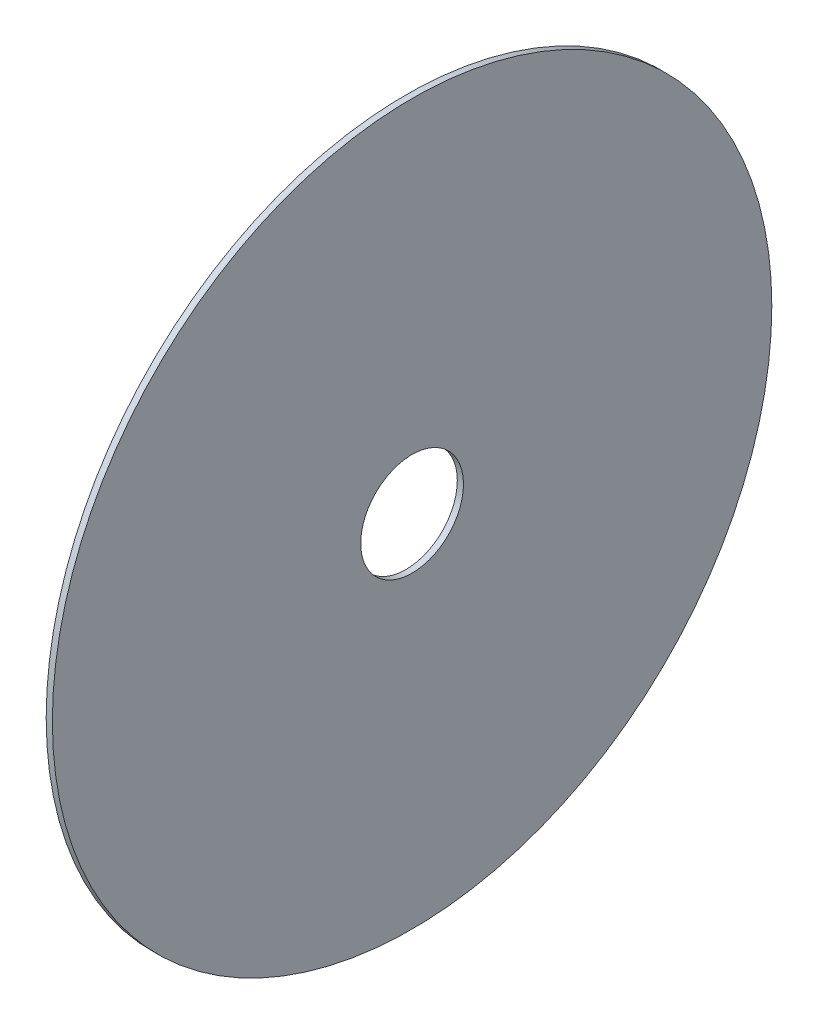
from build123d import *
from OCP.BRepFilletAPI import BRepFilletAPI_MakeChamfer

# Parameters (mm, degrees)
BOSS_EXTRUDE1_DEPTH = 4
CUT_EXTRUDE1_START  = -0.7
CUT_EXTRUDE1_DEPTH  = 0.7
CUT_EXTRUDE2_DEPTH  = 0.3
BOSS_EXTRUDE2_START = 0.3
BOSS_EXTRUDE2_DEPTH = 0.3
SKETCH5_W           = 3
SKETCH5_H           = 25
CHAMFER1_SIZE       = 1.130008551
CHAMFER1_SIZE2      = 0.565471506
SKETCH6_OUTSIDE_W   = 515.14
SKETCH6_OUTSIDE_H   = 515.14
SKETCH6_OUTSIDE_R   = 175
CUT_EXTRUDE3_DEPTH  = 10


with BuildPart() as part:
    # Sketch1 → Boss-Extrude1 (new body)
    with BuildSketch(Plane(origin=(-2, 0, 0), x_dir=(0, -1, 0), z_dir=(-1, 0, 0))):
        with BuildLine():
            Line((8.128598306, -199.834746453), (3.648717236, -192.075364828))
            ThreePointArc((3.648717236, -192.075364828), (3.941166203, -190.756212784), (5.280787083, -190.932577218))
            Line((5.280787083, -190.932577218), (12.558103906, -199.605345687))
            ThreePointArc((12.558103906, -199.605345687), (41.461654936, -195.655133258), (69.483089108, -187.54226278))
            Line((69.483089108, -187.54226278), (62.824688236, -181.547011706))
            ThreePointArc((62.824688236, -181.547011706), (62.695183332, -180.202051857), (64.023738106, -179.955818784))
            Line((64.023738106, -179.955818784), (73.624910537, -185.955297179))
            ThreePointArc((73.624910537, -185.955297179), (99.893138317, -173.266733442), (124.03609103, -156.891835741))
            Line((124.03609103, -156.891835741), (115.850941026, -153.247572166))
            ThreePointArc((115.850941026, -153.247572166), (115.312159093, -152.008458554), (116.499599564, -151.363730982))
            Line((116.499599564, -151.363730982), (127.48479795, -154.102648556))
            ThreePointArc((127.48479795, -154.102648556), (148.546385322, -133.917778536), (166.447576152, -110.883742691))
            Line((166.447576152, -110.883742691), (157.536896527, -109.947192524))
            ThreePointArc((157.536896527, -109.947192524), (156.641577295, -108.935218222), (157.571668516, -107.955106578))
            Line((157.571668516, -107.955106578), (168.8655851, -107.165358997))
            ThreePointArc((168.8655851, -107.165358997), (182.658877149, -81.460018407), (192.566012812, -54.021576334))
            Line((192.566012812, -54.021576334), (183.802042972, -55.88441563))
            ThreePointArc((183.802042972, -55.88441563), (182.637826525, -55.198639734), (183.219524688, -53.979084175))
            Line((183.219524688, -53.979084175), (193.716632226, -49.737977434))
            ThreePointArc((193.716632226, -49.737977434), (198.891445421, -21.028384111), (199.834746452, 8.128598305))
            Line((199.834746452, 8.128598305), (192.075364827, 3.648717235))
            ThreePointArc((192.075364827, 3.648717235), (190.756212783, 3.941166202), (190.932577217, 5.280787082))
            Line((190.932577217, 5.280787082), (199.605345686, 12.558103905))
            ThreePointArc((199.605345686, 12.558103905), (195.655133257, 41.461654935), (187.542262779, 69.483089106))
            Line((187.542262779, 69.483089106), (181.547011705, 62.824688235))
            ThreePointArc((181.547011705, 62.824688235), (180.202051856, 62.695183331), (179.955818783, 64.023738105))
            Line((179.955818783, 64.023738105), (185.955297178, 73.624910536))
            ThreePointArc((185.955297178, 73.624910536), (173.266733441, 99.893138316), (156.89183574, 124.036091029))
            Line((156.89183574, 124.036091029), (153.247572165, 115.850941024))
            ThreePointArc((153.247572165, 115.850941024), (152.008458553, 115.312159092), (151.363730981, 116.499599563))
            Line((151.363730981, 116.499599563), (154.102648555, 127.484797949))
            ThreePointArc((154.102648555, 127.484797949), (133.917778535, 148.546385321), (110.88374269, 166.447576151))
            Line((110.88374269, 166.447576151), (109.947192523, 157.536896526))
            ThreePointArc((109.947192523, 157.536896526), (108.935218221, 156.641577294), (107.955106577, 157.571668515))
            Line((107.955106577, 157.571668515), (107.165358996, 168.865585099))
            ThreePointArc((107.165358996, 168.865585099), (81.460018406, 182.658877148), (54.021576333, 192.566012811))
            Line((54.021576333, 192.566012811), (55.884415629, 183.802042971))
            ThreePointArc((55.884415629, 183.802042971), (55.198639733, 182.637826524), (53.979084174, 183.219524687))
            Line((53.979084174, 183.219524687), (49.737977433, 193.716632225))
            ThreePointArc((49.737977433, 193.716632225), (21.02838411, 198.89144542), (-8.128598306, 199.834746451))
            Line((-8.128598306, 199.834746451), (-3.648717236, 192.075364826))
            ThreePointArc((-3.648717236, 192.075364826), (-3.941166203, 190.756212782), (-5.280787083, 190.932577216))
            Line((-5.280787083, 190.932577216), (-12.558103906, 199.605345685))
            ThreePointArc((-12.558103906, 199.605345685), (-41.461654936, 195.655133256), (-69.483089107, 187.542262777))
            Line((-69.483089107, 187.542262777), (-62.824688236, 181.547011704))
            ThreePointArc((-62.824688236, 181.547011704), (-62.695183332, 180.202051855), (-64.023738106, 179.955818782))
            Line((-64.023738106, 179.955818782), (-73.624910537, 185.955297177))
            ThreePointArc((-73.624910537, 185.955297177), (-99.893138317, 173.26673344), (-124.03609103, 156.891835739))
            Line((-124.03609103, 156.891835739), (-115.850941025, 153.247572164))
            ThreePointArc((-115.850941025, 153.247572164), (-115.312159093, 152.008458552), (-116.499599564, 151.36373098))
            Line((-116.499599564, 151.36373098), (-127.48479795, 154.102648554))
            ThreePointArc((-127.48479795, 154.102648554), (-148.546385322, 133.917778533), (-166.447576152, 110.883742689))
            Line((-166.447576152, 110.883742689), (-157.536896527, 109.947192521))
            ThreePointArc((-157.536896527, 109.947192521), (-156.641577295, 108.93521822), (-157.571668516, 107.955106576))
            Line((-157.571668516, 107.955106576), (-168.8655851, 107.165358995))
            ThreePointArc((-168.8655851, 107.165358995), (-182.658877149, 81.460018404), (-192.566012812, 54.021576332))
            Line((-192.566012812, 54.021576332), (-183.802042972, 55.884415628))
            ThreePointArc((-183.802042972, 55.884415628), (-182.637826525, 55.198639732), (-183.219524688, 53.979084173))
            Line((-183.219524688, 53.979084173), (-193.716632226, 49.737977432))
            ThreePointArc((-193.716632226, 49.737977432), (-198.891445421, 21.028384109), (-199.834746452, -8.128598306))
            Line((-199.834746452, -8.128598306), (-192.075364827, -3.648717236))
            ThreePointArc((-192.075364827, -3.648717236), (-190.756212783, -3.941166203), (-190.932577217, -5.280787083))
            Line((-190.932577217, -5.280787083), (-199.605345686, -12.558103906))
            ThreePointArc((-199.605345686, -12.558103906), (-195.655133257, -41.461654937), (-187.542262778, -69.483089109))
            Line((-187.542262778, -69.483089109), (-181.547011705, -62.824688237))
            ThreePointArc((-181.547011705, -62.824688237), (-180.202051856, -62.695183333), (-179.955818783, -64.023738107))
            Line((-179.955818783, -64.023738107), (-185.955297178, -73.624910538))
            ThreePointArc((-185.955297178, -73.624910538), (-173.266733441, -99.893138318), (-156.89183574, -124.036091031))
            Line((-156.89183574, -124.036091031), (-153.247572165, -115.850941027))
            ThreePointArc((-153.247572165, -115.850941027), (-152.008458553, -115.312159094), (-151.363730981, -116.499599565))
            Line((-151.363730981, -116.499599565), (-154.102648555, -127.484797951))
            ThreePointArc((-154.102648555, -127.484797951), (-133.917778535, -148.546385324), (-110.88374269, -166.447576154))
            Line((-110.88374269, -166.447576154), (-109.947192522, -157.536896528))
            ThreePointArc((-109.947192522, -157.536896528), (-108.935218221, -156.641577296), (-107.955106577, -157.571668518))
            Line((-107.955106577, -157.571668518), (-107.165358996, -168.865585101))
            ThreePointArc((-107.165358996, -168.865585101), (-81.460018405, -182.65887715), (-54.021576333, -192.566012814))
            Line((-54.021576333, -192.566012814), (-55.884415629, -183.802042973))
            ThreePointArc((-55.884415629, -183.802042973), (-55.198639733, -182.637826526), (-53.979084174, -183.219524689))
            Line((-53.979084174, -183.219524689), (-49.737977433, -193.716632227))
            ThreePointArc((-49.737977433, -193.716632227), (-21.028384109, -198.891445422), (8.128598306, -199.834746453))
        make_face()
    extrude(amount=-BOSS_EXTRUDE1_DEPTH)

    # Sketch2 → Cut-Extrude1 (cut)
    with BuildSketch(Plane(origin=(2, 0, 0), x_dir=(0, 0, -1), z_dir=(1, 0, 0)).offset(CUT_EXTRUDE1_START)):
        with BuildLine():
            Line((181.547011705, -62.824688235), (181.845022607, -63.155662872))
            ThreePointArc((181.845022607, -63.155662872), (189.249413072, -35.226547542), (192.390100219, -6.503794095))
            Line((192.390100219, -6.503794095), (190.932577217, -5.280787082))
            ThreePointArc((190.932577217, -5.280787082), (190.756212783, -3.941166202), (192.075364827, -3.648717235))
            Line((192.075364827, -3.648717235), (192.461066825, -3.871402387))
            ThreePointArc((192.461066825, -3.871402387), (190.872489351, 24.978847229), (184.983641388, 53.266334763))
            Line((184.983641388, 53.266334763), (183.219524688, 53.979084175))
            ThreePointArc((183.219524688, 53.979084175), (182.637826525, 55.198639734), (183.802042972, 55.88441563))
            Line((183.802042972, 55.88441563), (184.237680867, 55.791817937))
            ThreePointArc((184.237680867, 55.791817937), (173.811636486, 82.739138395), (159.469694881, 107.822383645))
            Line((159.469694881, 107.822383645), (157.571668516, 107.955106578))
            ThreePointArc((157.571668516, 107.955106578), (156.641577295, 108.935218222), (157.536896527, 109.947192524))
            Line((157.536896527, 109.947192524), (157.979827047, 109.993746397))
            ThreePointArc((157.979827047, 109.993746397), (139.736889624, 132.400346217), (118.345743548, 151.824026374))
            Line((118.345743548, 151.824026374), (116.499599564, 151.363730982))
            ThreePointArc((116.499599564, 151.363730982), (115.312159093, 152.008458554), (115.850941025, 153.247572166))
            Line((115.850941025, 153.247572166), (116.257807045, 153.428720589))
            ThreePointArc((116.257807045, 153.428720589), (91.983722402, 169.101285665), (65.637286273, 180.964075582))
            Line((65.637286273, 180.964075582), (64.023738106, 179.955818784))
            ThreePointArc((64.023738106, 179.955818784), (62.695183332, 180.202051857), (62.824688236, 181.547011706))
            Line((62.824688236, 181.547011706), (63.155662873, 181.845022608))
            ThreePointArc((63.155662873, 181.845022608), (35.226547543, 189.249413073), (6.503794096, 192.39010022))
            Line((6.503794096, 192.39010022), (5.280787083, 190.932577218))
            ThreePointArc((5.280787083, 190.932577218), (3.941166203, 190.756212784), (3.648717236, 192.075364828))
            Line((3.648717236, 192.075364828), (3.871402389, 192.461066826))
            ThreePointArc((3.871402389, 192.461066826), (-24.978847228, 190.872489352), (-53.266334761, 184.983641389))
            Line((-53.266334761, 184.983641389), (-53.979084174, 183.219524689))
            ThreePointArc((-53.979084174, 183.219524689), (-55.198639733, 182.637826526), (-55.884415629, 183.802042973))
            Line((-55.884415629, 183.802042973), (-55.791817936, 184.237680869))
            ThreePointArc((-55.791817936, 184.237680869), (-82.739138394, 173.811636487), (-107.822383644, 159.469694882))
            Line((-107.822383644, 159.469694882), (-107.955106577, 157.571668518))
            ThreePointArc((-107.955106577, 157.571668518), (-108.935218221, 156.641577296), (-109.947192522, 157.536896528))
            Line((-109.947192522, 157.536896528), (-109.993746396, 157.979827048))
            ThreePointArc((-109.993746396, 157.979827048), (-132.400346216, 139.736889625), (-151.824026373, 118.345743549))
            Line((-151.824026373, 118.345743549), (-151.363730981, 116.499599565))
            ThreePointArc((-151.363730981, 116.499599565), (-152.008458553, 115.312159094), (-153.247572165, 115.850941027))
            Line((-153.247572165, 115.850941027), (-153.428720588, 116.257807046))
            ThreePointArc((-153.428720588, 116.257807046), (-169.101285664, 91.983722403), (-180.96407558, 65.637286274))
            Line((-180.96407558, 65.637286274), (-179.955818783, 64.023738107))
            ThreePointArc((-179.955818783, 64.023738107), (-180.202051856, 62.695183333), (-181.547011705, 62.824688237))
            Line((-181.547011705, 62.824688237), (-181.845022607, 63.155662874))
            ThreePointArc((-181.845022607, 63.155662874), (-189.249413072, 35.226547543), (-192.390100219, 6.503794096))
            Line((-192.390100219, 6.503794096), (-190.932577217, 5.280787083))
            ThreePointArc((-190.932577217, 5.280787083), (-190.756212783, 3.941166203), (-192.075364827, 3.648717236))
            Line((-192.075364827, 3.648717236), (-192.461066825, 3.871402388))
            ThreePointArc((-192.461066825, 3.871402388), (-190.872489351, -24.978847227), (-184.983641388, -53.26633476))
            Line((-184.983641388, -53.26633476), (-183.219524688, -53.979084173))
            ThreePointArc((-183.219524688, -53.979084173), (-182.637826525, -55.198639732), (-183.802042972, -55.884415628))
            Line((-183.802042972, -55.884415628), (-184.237680867, -55.791817935))
            ThreePointArc((-184.237680867, -55.791817935), (-173.811636486, -82.739138393), (-159.46969488, -107.822383643))
            Line((-159.46969488, -107.822383643), (-157.571668516, -107.955106576))
            ThreePointArc((-157.571668516, -107.955106576), (-156.641577295, -108.93521822), (-157.536896527, -109.947192521))
            Line((-157.536896527, -109.947192521), (-157.979827047, -109.993746395))
            ThreePointArc((-157.979827047, -109.993746395), (-139.736889624, -132.400346215), (-118.345743548, -151.824026372))
            Line((-118.345743548, -151.824026372), (-116.499599564, -151.36373098))
            ThreePointArc((-116.499599564, -151.36373098), (-115.312159093, -152.008458552), (-115.850941025, -153.247572164))
            Line((-115.850941025, -153.247572164), (-116.257807045, -153.428720587))
            ThreePointArc((-116.257807045, -153.428720587), (-91.983722402, -169.101285663), (-65.637286273, -180.964075579))
            Line((-65.637286273, -180.964075579), (-64.023738106, -179.955818782))
            ThreePointArc((-64.023738106, -179.955818782), (-62.695183332, -180.202051855), (-62.824688236, -181.547011704))
            Line((-62.824688236, -181.547011704), (-63.155662873, -181.845022606))
            ThreePointArc((-63.155662873, -181.845022606), (-35.226547543, -189.249413071), (-6.503794096, -192.390100218))
            Line((-6.503794096, -192.390100218), (-5.280787083, -190.932577216))
            ThreePointArc((-5.280787083, -190.932577216), (-3.941166203, -190.756212782), (-3.648717236, -192.075364826))
            Line((-3.648717236, -192.075364826), (-3.871402388, -192.461066824))
            ThreePointArc((-3.871402388, -192.461066824), (24.978847228, -190.87248935), (53.266334762, -184.983641387))
            Line((53.266334762, -184.983641387), (53.979084174, -183.219524687))
            ThreePointArc((53.979084174, -183.219524687), (55.198639733, -182.637826524), (55.884415629, -183.802042971))
            Line((55.884415629, -183.802042971), (55.791817936, -184.237680866))
            ThreePointArc((55.791817936, -184.237680866), (82.739138394, -173.811636485), (107.822383644, -159.469694879))
            Line((107.822383644, -159.469694879), (107.955106577, -157.571668515))
            ThreePointArc((107.955106577, -157.571668515), (108.935218221, -156.641577294), (109.947192523, -157.536896526))
            Line((109.947192523, -157.536896526), (109.993746396, -157.979827046))
            ThreePointArc((109.993746396, -157.979827046), (132.400346216, -139.736889623), (151.824026373, -118.345743546))
            Line((151.824026373, -118.345743546), (151.363730981, -116.499599563))
            ThreePointArc((151.363730981, -116.499599563), (152.008458553, -115.312159092), (153.247572165, -115.850941024))
            Line((153.247572165, -115.850941024), (153.428720588, -116.257807044))
            ThreePointArc((153.428720588, -116.257807044), (169.101285664, -91.983722401), (180.964075581, -65.637286272))
            Line((180.964075581, -65.637286272), (179.955818783, -64.023738105))
            ThreePointArc((179.955818783, -64.023738105), (180.202051856, -62.695183331), (181.547011705, -62.824688235))
        make_face()
    extrude(amount=CUT_EXTRUDE1_DEPTH, mode=Mode.SUBTRACT)

    # Sketch3 → Cut-Extrude2 (cut)
    with BuildSketch(Plane.ZY.offset(2)):
        with BuildLine():
            Line((-190.932577217, -5.280787083), (-199.605345686, -12.558103906))
            ThreePointArc((-199.605345686, -12.558103906), (-195.655133257, -41.461654936), (-187.542262779, -69.483089108))
            Line((-187.542262779, -69.483089108), (-181.547011705, -62.824688236))
            ThreePointArc((-181.547011705, -62.824688236), (-180.202051856, -62.695183332), (-179.955818783, -64.023738106))
            Line((-179.955818783, -64.023738106), (-180.964075581, -65.637286273))
            ThreePointArc((-180.964075581, -65.637286273), (-169.101285664, -91.983722402), (-153.428720588, -116.257807045))
            Line((-153.428720588, -116.257807045), (-153.247572165, -115.850941025))
            ThreePointArc((-153.247572165, -115.850941025), (-152.008458553, -115.312159093), (-151.363730981, -116.499599564))
            Line((-151.363730981, -116.499599564), (-151.824026373, -118.345743548))
            ThreePointArc((-151.824026373, -118.345743548), (-132.400346216, -139.736889624), (-109.993746396, -157.979827047))
            Line((-109.993746396, -157.979827047), (-109.947192522, -157.536896527))
            ThreePointArc((-109.947192522, -157.536896527), (-108.935218221, -156.641577295), (-107.955106577, -157.571668516))
            Line((-107.955106577, -157.571668516), (-107.822383644, -159.46969488))
            ThreePointArc((-107.822383644, -159.46969488), (-82.739138394, -173.811636486), (-55.791817936, -184.237680867))
            Line((-55.791817936, -184.237680867), (-55.884415629, -183.802042972))
            ThreePointArc((-55.884415629, -183.802042972), (-55.198639733, -182.637826525), (-53.979084174, -183.219524688))
            Line((-53.979084174, -183.219524688), (-53.266334761, -184.983641388))
            ThreePointArc((-53.266334761, -184.983641388), (-24.978847228, -190.872489351), (3.871402388, -192.461066825))
            Line((3.871402388, -192.461066825), (3.648717236, -192.075364827))
            ThreePointArc((3.648717236, -192.075364827), (3.941166203, -190.756212783), (5.280787083, -190.932577217))
            Line((5.280787083, -190.932577217), (6.503794096, -192.390100219))
            ThreePointArc((6.503794096, -192.390100219), (35.226547543, -189.249413072), (63.155662873, -181.845022607))
            Line((63.155662873, -181.845022607), (62.824688236, -181.547011705))
            ThreePointArc((62.824688236, -181.547011705), (62.695183332, -180.202051856), (64.023738106, -179.955818783))
            Line((64.023738106, -179.955818783), (65.637286273, -180.964075581))
            ThreePointArc((65.637286273, -180.964075581), (91.983722402, -169.101285664), (116.257807045, -153.428720588))
            Line((116.257807045, -153.428720588), (115.850941025, -153.247572165))
            ThreePointArc((115.850941025, -153.247572165), (115.312159093, -152.008458553), (116.499599564, -151.363730981))
            Line((116.499599564, -151.363730981), (118.345743548, -151.824026373))
            ThreePointArc((118.345743548, -151.824026373), (139.736889624, -132.400346216), (157.979827047, -109.993746396))
            Line((157.979827047, -109.993746396), (157.536896527, -109.947192522))
            ThreePointArc((157.536896527, -109.947192522), (156.641577295, -108.935218221), (157.571668516, -107.955106577))
            Line((157.571668516, -107.955106577), (159.46969488, -107.822383644))
            ThreePointArc((159.46969488, -107.822383644), (173.811636486, -82.739138394), (184.237680867, -55.791817936))
            Line((184.237680867, -55.791817936), (183.802042972, -55.884415629))
            ThreePointArc((183.802042972, -55.884415629), (182.637826525, -55.198639733), (183.219524688, -53.979084174))
            Line((183.219524688, -53.979084174), (184.983641388, -53.266334761))
            ThreePointArc((184.983641388, -53.266334761), (190.872489351, -24.978847228), (192.461066825, 3.871402388))
            Line((192.461066825, 3.871402388), (192.075364827, 3.648717236))
            ThreePointArc((192.075364827, 3.648717236), (190.756212783, 3.941166203), (190.932577217, 5.280787083))
            Line((190.932577217, 5.280787083), (192.390100219, 6.503794096))
            ThreePointArc((192.390100219, 6.503794096), (189.249413072, 35.226547543), (181.845022607, 63.155662873))
            Line((181.845022607, 63.155662873), (181.547011705, 62.824688236))
            ThreePointArc((181.547011705, 62.824688236), (180.202051856, 62.695183332), (179.955818783, 64.023738106))
            Line((179.955818783, 64.023738106), (180.964075581, 65.637286273))
            ThreePointArc((180.964075581, 65.637286273), (169.101285664, 91.983722402), (153.428720588, 116.257807045))
            Line((153.428720588, 116.257807045), (153.247572165, 115.850941025))
            ThreePointArc((153.247572165, 115.850941025), (152.008458553, 115.312159093), (151.363730981, 116.499599564))
            Line((151.363730981, 116.499599564), (151.824026373, 118.345743548))
            ThreePointArc((151.824026373, 118.345743548), (132.400346216, 139.736889624), (109.993746396, 157.979827047))
            Line((109.993746396, 157.979827047), (109.947192522, 157.536896527))
            ThreePointArc((109.947192522, 157.536896527), (108.935218221, 156.641577295), (107.955106577, 157.571668516))
            Line((107.955106577, 157.571668516), (107.822383644, 159.46969488))
            ThreePointArc((107.822383644, 159.46969488), (82.739138394, 173.811636486), (55.791817936, 184.237680867))
            Line((55.791817936, 184.237680867), (55.884415629, 183.802042972))
            ThreePointArc((55.884415629, 183.802042972), (55.198639733, 182.637826525), (53.979084174, 183.219524688))
            Line((53.979084174, 183.219524688), (53.266334761, 184.983641388))
            ThreePointArc((53.266334761, 184.983641388), (24.978847228, 190.872489351), (-3.871402388, 192.461066825))
            Line((-3.871402388, 192.461066825), (-3.648717236, 192.075364827))
            ThreePointArc((-3.648717236, 192.075364827), (-3.941166203, 190.756212783), (-5.280787083, 190.932577217))
            Line((-5.280787083, 190.932577217), (-6.503794096, 192.390100219))
            ThreePointArc((-6.503794096, 192.390100219), (-35.226547543, 189.249413072), (-63.155662873, 181.845022607))
            Line((-63.155662873, 181.845022607), (-62.824688236, 181.547011705))
            ThreePointArc((-62.824688236, 181.547011705), (-62.695183332, 180.202051856), (-64.023738106, 179.955818783))
            Line((-64.023738106, 179.955818783), (-65.637286273, 180.964075581))
            ThreePointArc((-65.637286273, 180.964075581), (-91.983722402, 169.101285664), (-116.257807045, 153.428720588))
            Line((-116.257807045, 153.428720588), (-115.850941025, 153.247572165))
            ThreePointArc((-115.850941025, 153.247572165), (-115.312159093, 152.008458553), (-116.499599564, 151.363730981))
            Line((-116.499599564, 151.363730981), (-118.345743548, 151.824026373))
            ThreePointArc((-118.345743548, 151.824026373), (-139.736889624, 132.400346216), (-157.979827047, 109.993746396))
            Line((-157.979827047, 109.993746396), (-157.536896527, 109.947192522))
            ThreePointArc((-157.536896527, 109.947192522), (-156.641577295, 108.935218221), (-157.571668516, 107.955106577))
            Line((-157.571668516, 107.955106577), (-159.46969488, 107.822383644))
            ThreePointArc((-159.46969488, 107.822383644), (-173.811636486, 82.739138394), (-184.237680867, 55.791817936))
            Line((-184.237680867, 55.791817936), (-183.802042972, 55.884415629))
            ThreePointArc((-183.802042972, 55.884415629), (-182.637826525, 55.198639733), (-183.219524688, 53.979084174))
            Line((-183.219524688, 53.979084174), (-184.983641388, 53.266334761))
            ThreePointArc((-184.983641388, 53.266334761), (-190.872489351, 24.978847228), (-192.461066825, -3.871402388))
            Line((-192.461066825, -3.871402388), (-192.075364827, -3.648717236))
            ThreePointArc((-192.075364827, -3.648717236), (-190.756212783, -3.941166203), (-190.932577217, -5.280787083))
        make_face()
    extrude(amount=-CUT_EXTRUDE2_DEPTH, mode=Mode.SUBTRACT)

    # Sketch4 → Boss-Extrude2 (add)
    with BuildSketch(Plane.ZY.offset(1.7).offset(BOSS_EXTRUDE2_START)):
        with BuildLine():
            Line((-199.605345686, -12.558103906), (-192.390100219, -6.503794096))
            ThreePointArc((-192.390100219, -6.503794096), (-189.249413072, -35.226547543), (-181.845022607, -63.155662873))
            Line((-181.845022607, -63.155662873), (-187.542262779, -69.483089108))
            ThreePointArc((-187.542262779, -69.483089108), (-195.655133257, -41.461654936), (-199.605345686, -12.558103906))
        make_face()
    extrude(amount=-BOSS_EXTRUDE2_DEPTH)

    # Sketch5 → Cut-Revolve1 (revolve, cut)
    with BuildSketch(Plane.XY, mode=Mode.PRIVATE) as cut_revolve1_sk:
        with Locations((-0.2, 12.5)):
            Rectangle(SKETCH5_W, SKETCH5_H)
    revolve(cut_revolve1_sk.sketch.rotate(Axis((-1.7, 0, 0), (1, 0, 0)), 270), axis=Axis((-1.7, 0, 0), (1, 0, 0)), mode=Mode.SUBTRACT)

    # Chamfer1: one chamfer whose edges measure the first distance from different faces: ONE call of the kernel's chamfer builder (chamfer() names one face for all edges)
    chamfer1_edges_1 = [part.edges().sort_by_distance(p)[0] for p in [
        (0, 54.021576333, -192.566012814),
    ]]
    chamfer1_side_1 = [part.faces().sort_by_distance(p)[0] for p in [
        (-0.007549997, 54.941858215, -188.236426965),
    ]]
    chamfer1_edges_2 = [part.edges().sort_by_distance(p)[0] for p in [
        (0, 110.88374269, -166.447576154),
    ]]
    chamfer1_side_2 = [part.faces().sort_by_distance(p)[0] for p in [
        (-0.007549998, 110.421067164, -162.045512578),
    ]]
    chamfer1_edges_3 = [part.edges().sort_by_distance(p)[0] for p in [
        (0, 156.89183574, -124.036091031),
    ]]
    chamfer1_side_3 = [part.faces().sort_by_distance(p)[0] for p in [
        (-0.007549998, 155.091492712, -119.992454383),
    ]]
    chamfer1_edges_4 = [part.edges().sort_by_distance(p)[0] for p in [
        (0, 187.542262778, -69.483089109),
    ]]
    chamfer1_side_4 = [part.faces().sort_by_distance(p)[0] for p in [
        (-0.007549998, 184.580482366, -66.193698716),
    ]]
    chamfer1_edges_5 = [part.edges().sort_by_distance(p)[0] for p in [
        (0, 199.834746452, -8.128598306),
    ]]
    chamfer1_side_5 = [part.faces().sort_by_distance(p)[0] for p in [
        (-0.007549998, 196.001448359, -5.91544262),
    ]]
    chamfer1_edges_6 = [part.edges().sort_by_distance(p)[0] for p in [
        (0, 192.566012812, 54.021576332),
    ]]
    chamfer1_side_6 = [part.faces().sort_by_distance(p)[0] for p in [
        (-0.007549998, 188.236426964, 54.941858214),
    ]]
    chamfer1_edges_7 = [part.edges().sort_by_distance(p)[0] for p in [
        (0, 166.447576152, 110.883742689),
    ]]
    chamfer1_side_7 = [part.faces().sort_by_distance(p)[0] for p in [
        (-0.007549998, 162.045512577, 110.421067163),
    ]]
    chamfer1_edges_8 = [part.edges().sort_by_distance(p)[0] for p in [
        (0, 124.03609103, 156.891835739),
    ]]
    chamfer1_side_8 = [part.faces().sort_by_distance(p)[0] for p in [
        (-0.007549998, 119.992454382, 155.091492711),
    ]]
    chamfer1_edges_9 = [part.edges().sort_by_distance(p)[0] for p in [
        (0, 69.483089107, 187.542262777),
    ]]
    chamfer1_side_9 = [part.faces().sort_by_distance(p)[0] for p in [
        (-0.007549998, 66.193698715, 184.580482365),
    ]]
    chamfer1_edges_10 = [part.edges().sort_by_distance(p)[0] for p in [
        (0, 8.128598306, 199.834746451),
    ]]
    chamfer1_side_10 = [part.faces().sort_by_distance(p)[0] for p in [
        (-0.007549998, 5.91544262, 196.001448358),
    ]]
    chamfer1_edges_11 = [part.edges().sort_by_distance(p)[0] for p in [
        (0, -54.021576333, 192.566012811),
    ]]
    chamfer1_side_11 = [part.faces().sort_by_distance(p)[0] for p in [
        (-0.007549998, -54.941858215, 188.236426963),
    ]]
    chamfer1_edges_12 = [part.edges().sort_by_distance(p)[0] for p in [
        (0, -110.88374269, 166.447576151),
    ]]
    chamfer1_side_12 = [part.faces().sort_by_distance(p)[0] for p in [
        (-0.007549998, -110.421067165, 162.045512576),
    ]]
    chamfer1_edges_13 = [part.edges().sort_by_distance(p)[0] for p in [
        (0, -156.89183574, 124.036091029),
    ]]
    chamfer1_side_13 = [part.faces().sort_by_distance(p)[0] for p in [
        (-0.007549998, -155.091492712, 119.992454381),
    ]]
    chamfer1_edges_14 = [part.edges().sort_by_distance(p)[0] for p in [
        (0, -187.542262779, 69.483089106),
    ]]
    chamfer1_side_14 = [part.faces().sort_by_distance(p)[0] for p in [
        (-0.007549998, -184.580482366, 66.193698714),
    ]]
    chamfer1_edges_15 = [part.edges().sort_by_distance(p)[0] for p in [
        (0, -199.834746452, 8.128598305),
    ]]
    chamfer1_side_15 = [part.faces().sort_by_distance(p)[0] for p in [
        (-0.007549997, -196.001448359, 5.915442619),
    ]]
    chamfer1_edges_16 = [part.edges().sort_by_distance(p)[0] for p in [
        (0, -192.566012812, -54.021576334),
    ]]
    chamfer1_side_16 = [part.faces().sort_by_distance(p)[0] for p in [
        (-0.007549997, -188.236426964, -54.941858216),
    ]]
    chamfer1_edges_17 = [part.edges().sort_by_distance(p)[0] for p in [
        (0, -166.447576152, -110.883742691),
    ]]
    chamfer1_side_17 = [part.faces().sort_by_distance(p)[0] for p in [
        (-0.007549997, -162.045512577, -110.421067166),
    ]]
    chamfer1_edges_18 = [part.edges().sort_by_distance(p)[0] for p in [
        (0, -124.03609103, -156.891835741),
    ]]
    chamfer1_side_18 = [part.faces().sort_by_distance(p)[0] for p in [
        (-0.007549997, -119.992454382, -155.091492713),
    ]]
    chamfer1_edges_19 = [part.edges().sort_by_distance(p)[0] for p in [
        (0.15, -69.483089108, -187.54226278),
    ]]
    chamfer1_side_19 = [part.faces().sort_by_distance(p)[0] for p in [
        (-0.007549997, -66.193698715, -184.580482367),
    ]]
    chamfer1_edges_20 = [part.edges().sort_by_distance(p)[0] for p in [
        (0, -8.128598306, -199.834746453),
    ]]
    chamfer1_side_20 = [part.faces().sort_by_distance(p)[0] for p in [
        (-0.007549997, -5.91544262, -196.00144836),
    ]]
    chamfer1 = BRepFilletAPI_MakeChamfer(part.part.solid().wrapped)
    for e in chamfer1_edges_1:
        chamfer1.Add(CHAMFER1_SIZE, CHAMFER1_SIZE2, e.wrapped, chamfer1_side_1[0].wrapped)  # the first distance lies on this face
    for e in chamfer1_edges_2:
        chamfer1.Add(CHAMFER1_SIZE, CHAMFER1_SIZE2, e.wrapped, chamfer1_side_2[0].wrapped)  # the first distance lies on this face
    for e in chamfer1_edges_3:
        chamfer1.Add(CHAMFER1_SIZE, CHAMFER1_SIZE2, e.wrapped, chamfer1_side_3[0].wrapped)  # the first distance lies on this face
    for e in chamfer1_edges_4:
        chamfer1.Add(CHAMFER1_SIZE, CHAMFER1_SIZE2, e.wrapped, chamfer1_side_4[0].wrapped)  # the first distance lies on this face
    for e in chamfer1_edges_5:
        chamfer1.Add(CHAMFER1_SIZE, CHAMFER1_SIZE2, e.wrapped, chamfer1_side_5[0].wrapped)  # the first distance lies on this face
    for e in chamfer1_edges_6:
        chamfer1.Add(CHAMFER1_SIZE, CHAMFER1_SIZE2, e.wrapped, chamfer1_side_6[0].wrapped)  # the first distance lies on this face
    for e in chamfer1_edges_7:
        chamfer1.Add(CHAMFER1_SIZE, CHAMFER1_SIZE2, e.wrapped, chamfer1_side_7[0].wrapped)  # the first distance lies on this face
    for e in chamfer1_edges_8:
        chamfer1.Add(CHAMFER1_SIZE, CHAMFER1_SIZE2, e.wrapped, chamfer1_side_8[0].wrapped)  # the first distance lies on this face
    for e in chamfer1_edges_9:
        chamfer1.Add(CHAMFER1_SIZE, CHAMFER1_SIZE2, e.wrapped, chamfer1_side_9[0].wrapped)  # the first distance lies on this face
    for e in chamfer1_edges_10:
        chamfer1.Add(CHAMFER1_SIZE, CHAMFER1_SIZE2, e.wrapped, chamfer1_side_10[0].wrapped)  # the first distance lies on this face
    for e in chamfer1_edges_11:
        chamfer1.Add(CHAMFER1_SIZE, CHAMFER1_SIZE2, e.wrapped, chamfer1_side_11[0].wrapped)  # the first distance lies on this face
    for e in chamfer1_edges_12:
        chamfer1.Add(CHAMFER1_SIZE, CHAMFER1_SIZE2, e.wrapped, chamfer1_side_12[0].wrapped)  # the first distance lies on this face
    for e in chamfer1_edges_13:
        chamfer1.Add(CHAMFER1_SIZE, CHAMFER1_SIZE2, e.wrapped, chamfer1_side_13[0].wrapped)  # the first distance lies on this face
    for e in chamfer1_edges_14:
        chamfer1.Add(CHAMFER1_SIZE, CHAMFER1_SIZE2, e.wrapped, chamfer1_side_14[0].wrapped)  # the first distance lies on this face
    for e in chamfer1_edges_15:
        chamfer1.Add(CHAMFER1_SIZE, CHAMFER1_SIZE2, e.wrapped, chamfer1_side_15[0].wrapped)  # the first distance lies on this face
    for e in chamfer1_edges_16:
        chamfer1.Add(CHAMFER1_SIZE, CHAMFER1_SIZE2, e.wrapped, chamfer1_side_16[0].wrapped)  # the first distance lies on this face
    for e in chamfer1_edges_17:
        chamfer1.Add(CHAMFER1_SIZE, CHAMFER1_SIZE2, e.wrapped, chamfer1_side_17[0].wrapped)  # the first distance lies on this face
    for e in chamfer1_edges_18:
        chamfer1.Add(CHAMFER1_SIZE, CHAMFER1_SIZE2, e.wrapped, chamfer1_side_18[0].wrapped)  # the first distance lies on this face
    for e in chamfer1_edges_19:
        chamfer1.Add(CHAMFER1_SIZE, CHAMFER1_SIZE2, e.wrapped, chamfer1_side_19[0].wrapped)  # the first distance lies on this face
    for e in chamfer1_edges_20:
        chamfer1.Add(CHAMFER1_SIZE, CHAMFER1_SIZE2, e.wrapped, chamfer1_side_20[0].wrapped)  # the first distance lies on this face
    add(Compound.cast(chamfer1.Shape()), mode=Mode.REPLACE)

    # Sketch6 outside → Cut-Extrude3 (cut)
    with BuildSketch(Plane.ZY.offset(2)):
        Rectangle(SKETCH6_OUTSIDE_W, SKETCH6_OUTSIDE_H)
        Circle(SKETCH6_OUTSIDE_R, mode=Mode.SUBTRACT)
    extrude(amount=-CUT_EXTRUDE3_DEPTH, mode=Mode.SUBTRACT)


solid = part.part
